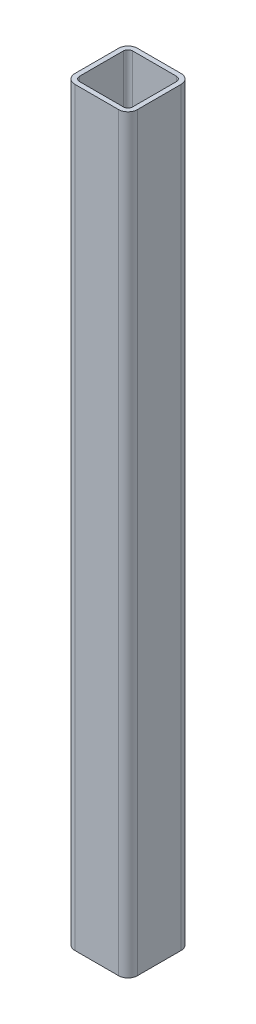
from build123d import *

# Parameters (mm, degrees)
COLD_FORMED_HOLLOW_SQUARE_STEEL_GB_T672_DEPTH = 480


with BuildPart() as part:
    # Sketch12 → Cold-formed hollow square steel (gb t6728-2002) 40×3-example.com(1) (new body)
    with BuildSketch(Plane(origin=(0, 0, 0), x_dir=(-1, 0, 0), z_dir=(0, 1, 0))):
        with BuildLine():
            Line((-14, -20), (14, -20))
            ThreePointArc((14, -20), (18.242640687, -18.242640687), (20, -14))
            Line((20, -14), (20, 14))
            ThreePointArc((20, 14), (18.242640687, 18.242640687), (14, 20))
            Line((14, 20), (-14, 20))
            ThreePointArc((-14, 20), (-18.242640687, 18.242640687), (-20, 14))
            Line((-20, 14), (-20, -14))
            ThreePointArc((-20, -14), (-18.242640687, -18.242640687), (-14, -20))
        make_face()
        with BuildLine():
            Line((-14, -17), (14, -17))
            ThreePointArc((14, -17), (16.121320344, -16.121320344), (17, -14))
            Line((17, -14), (17, 14))
            ThreePointArc((17, 14), (16.121320344, 16.121320344), (14, 17))
            Line((14, 17), (-14, 17))
            ThreePointArc((-14, 17), (-16.121320344, 16.121320344), (-17, 14))
            Line((-17, 14), (-17, -14))
            ThreePointArc((-17, -14), (-16.121320344, -16.121320344), (-14, -17))
        make_face(mode=Mode.SUBTRACT)
    extrude(amount=COLD_FORMED_HOLLOW_SQUARE_STEEL_GB_T672_DEPTH)


solid = part.part
